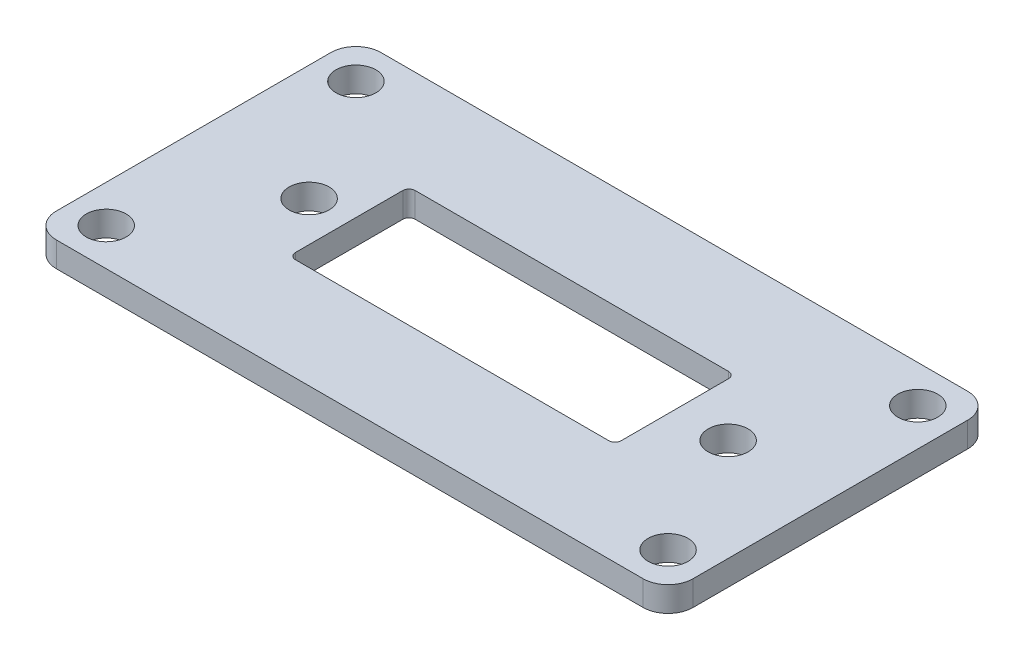
from build123d import *

# Parameters (mm, degrees)
SKETCH1_R           = 1.6
BOSS_EXTRUDE1_DEPTH = 2
SKETCH2_R           = 1.6
SKETCH2_W           = 26.1
SKETCH2_H           = 9.6
CUT_EXTRUDE1_DEPTH  = 2
FILLET1_R           = 0.5


with BuildPart() as part:
    # Sketch1 → Boss-Extrude1 (new body)
    with BuildSketch(Plane(origin=(0, 0, 0), x_dir=(1, 0, 0), z_dir=(0, 1, 0))):
        with BuildLine():
            Line((-23.5, -13), (23.5, -13))
            ThreePointArc((23.5, -13), (24.914213562, -12.414213562), (25.5, -11))
            Line((25.5, -11), (25.5, 11))
            ThreePointArc((25.5, 11), (24.914213562, 12.414213562), (23.5, 13))
            Line((23.5, 13), (-23.5, 13))
            ThreePointArc((-23.5, 13), (-24.914213562, 12.414213562), (-25.5, 11))
            Line((-25.5, 11), (-25.5, -11))
            ThreePointArc((-25.5, -11), (-24.914213562, -12.414213562), (-23.5, -13))
        make_face()
        with Locations(Location((-22.5, 10, 0), (0, 0, 270))):
            Circle(SKETCH1_R, mode=Mode.SUBTRACT)
        with Locations(Location((22.5, 10, 0), (0, 0, 270))):
            Circle(SKETCH1_R, mode=Mode.SUBTRACT)
        with Locations(Location((22.5, -10, 0), (0, 0, 270))):
            Circle(SKETCH1_R, mode=Mode.SUBTRACT)
        with Locations(Location((-22.5, -10, 0), (0, 0, 270))):
            Circle(SKETCH1_R, mode=Mode.SUBTRACT)
    extrude(amount=BOSS_EXTRUDE1_DEPTH)

    # Sketch2 → Cut-Extrude1 (cut)
    with BuildSketch(Plane.XZ):
        with Locations(Location((-16.25, 0, 0), (0, 0, 270))):
            Circle(SKETCH2_R)
        with Locations(Location((17.311344744, 0, 0), (0, 0, 270))):
            Circle(SKETCH2_R)
        Rectangle(SKETCH2_W, SKETCH2_H)
    extrude(amount=-CUT_EXTRUDE1_DEPTH, mode=Mode.SUBTRACT)

    # Fillet1
    fillet1_edges = [part.edges().sort_by_distance(p)[0] for p in [
        (13.05, 1, 4.8),
        (13.05, 1, -4.8),
        (-13.05, 1, -4.8),
        (-13.05, 1, 4.8),
    ]]
    fillet(fillet1_edges, radius=FILLET1_R)


solid = part.part
